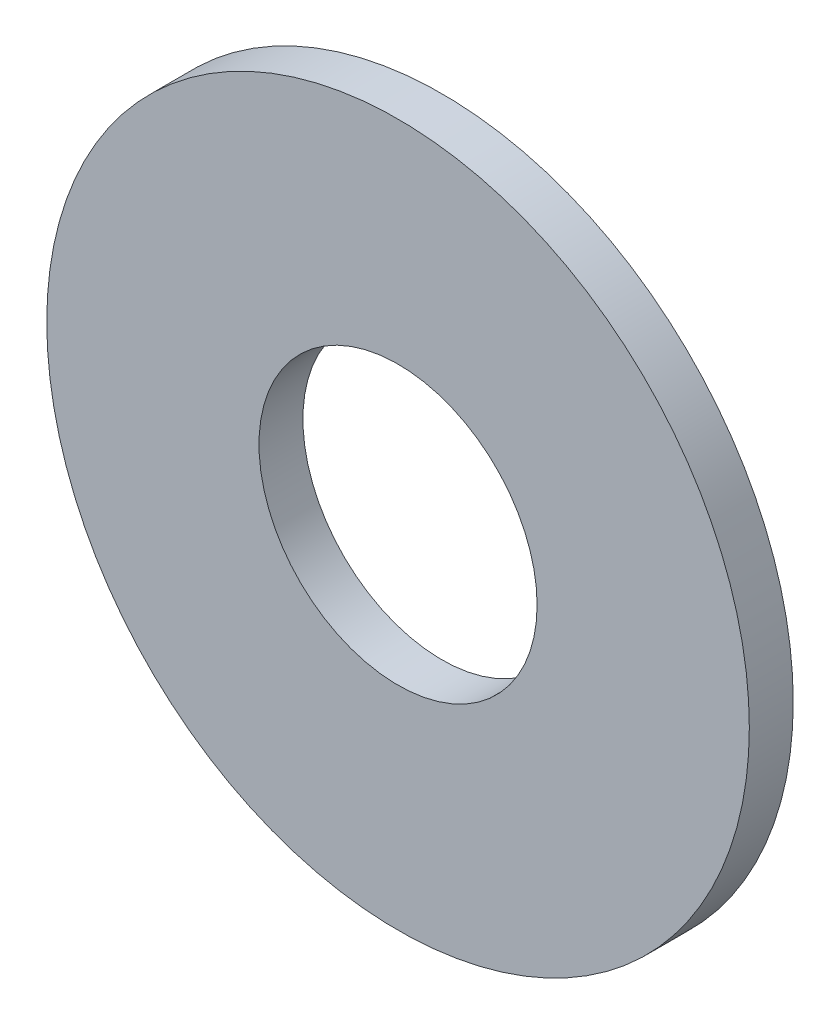
SolidWorks part; units mm, degrees
ref_plane "Front Plane" through (0, 0, 0) normal (0, 0, 1) x (1, 0, 0)
ref_plane "Top Plane" through (0, 0, 0) normal (0, 1, 0) x (1, 0, 0)
ref_plane "Right Plane" through (0, 0, 0) normal (1, 0, 0) x (0, 0, -1)
sketch "Sketch1" plane through (0, 0, 0) normal (0, 0, 1) x (1, 0, 0)
  circle A0 centre (0, 0) radius 9.5
  circle A1 centre (0, 0) radius 24
  dimension "D1" = 19
  dimension "D2" = 48
extrude "Extrude1" add sketch "Sketch1" along normal blind 3
